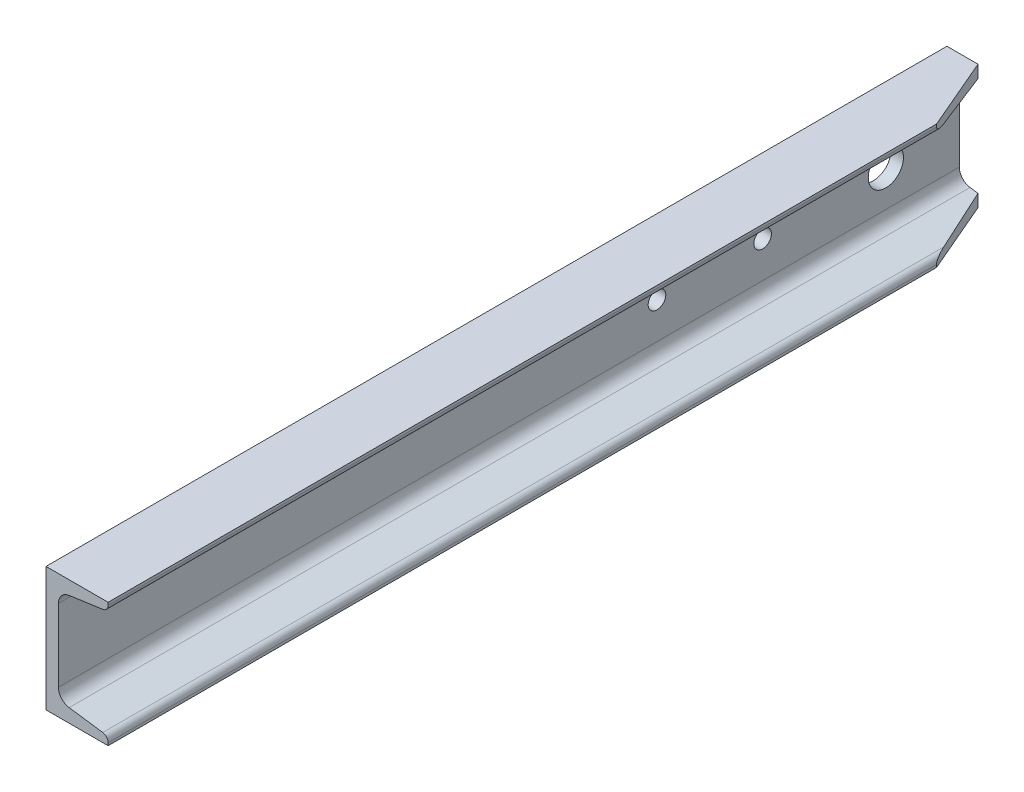
from build123d import *

# Parameters (mm, degrees)
BOSS_EXTRUDE1_DEPTH = 435
SKETCH2_R           = 8.5
CUT_EXTRUDE1_DEPTH  = 435
CUT_EXTRUDE2_DEPTH  = 435
SKETCH4_R           = 4.25
CUT_EXTRUDE3_DEPTH  = 435


with BuildPart() as part:
    # Sketch1 → Boss-Extrude1 (new body)
    with BuildSketch(Plane.XY):
        with BuildLine():
            Line((0, 0), (-30, 0))
            Line((-30, 0), (-30, -60))
            Line((-30, -60), (0, -60))
            Line((0, -60), (0, -58.715972734))
            ThreePointArc((0, -58.715972734), (-0.735871259, -56.747795647), (-2.582480697, -55.745168528))
            Line((-2.582480697, -55.745168528), (-18.835038606, -53.461020473))
            ThreePointArc((-18.835038606, -53.461020473), (-22.528257481, -51.455766235), (-24, -47.519412061))
            Line((-24, -47.519412061), (-24, -12.480587939))
            ThreePointArc((-24, -12.480587939), (-22.528257481, -8.544233765), (-18.835038606, -6.538979527))
            Line((-18.835038606, -6.538979527), (-2.582480697, -4.254831472))
            ThreePointArc((-2.582480697, -4.254831472), (-0.735871259, -3.252204353), (0, -1.284027266))
            Line((0, -1.284027266), (0, 0))
        make_face()
    extrude(amount=BOSS_EXTRUDE1_DEPTH)

    # Sketch2 → Cut-Extrude1 (cut)
    with BuildSketch(Plane.ZY.offset(30)):
        with Locations(Location((35.5, -30, 0), (0, 0, 270))):
            Circle(SKETCH2_R)
    extrude(amount=-CUT_EXTRUDE1_DEPTH, mode=Mode.SUBTRACT)

    # Sketch3 → Cut-Extrude2 (cut)
    with BuildSketch(Plane(origin=(0, 0, 0), x_dir=(1, 0, 0), z_dir=(0, 1, 0))):
        Polygon((-15, 0), (0, 0), (0, -35), align=None)
    extrude(amount=-CUT_EXTRUDE2_DEPTH, mode=Mode.SUBTRACT)

    # Sketch4 → Cut-Extrude3 (cut)
    with BuildSketch(Plane.ZY.offset(30)):
        with Locations(Location((95, -30, 0), (0, 0, 270))):
            Circle(SKETCH4_R)
        with Locations(Location((146, -30, 0), (0, 0, 270))):
            Circle(SKETCH4_R)
    extrude(amount=-CUT_EXTRUDE3_DEPTH, mode=Mode.SUBTRACT)


solid = part.part
